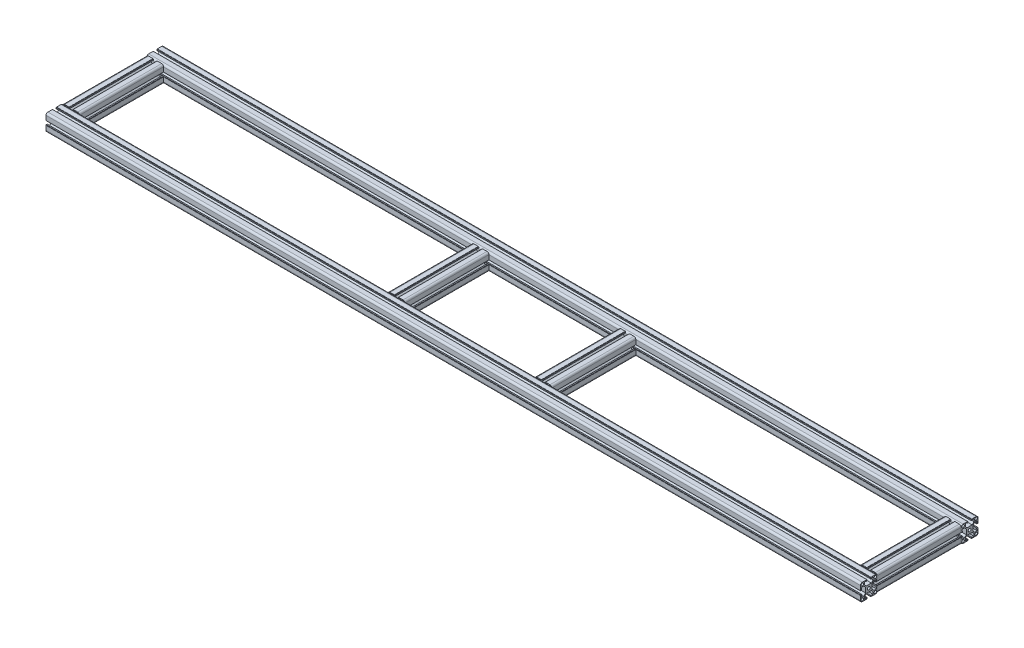
from build123d import *

# Parameters (mm, degrees)
F_40_X_40W_X_R4_5_1_DEPTH      = 1920
F_40_X_40W_X_R4_5_1_DEPTH_BACK = 20
SKETCH1_R                      = 3.4
SKETCH1_R_2                    = 3
SKETCH1_ON_SEGMENT_2_R         = 3.4
SKETCH1_ON_SEGMENT_2_R_2       = 3
F_40_X_40W_X_R4_5_1_2_DEPTH    = 1940
SKETCH1_ON_SEGMENT_3_R         = 3.4
SKETCH1_ON_SEGMENT_3_R_2       = 3
F_40_X_40W_X_R4_5_1_3_DEPTH    = 242
SKETCH1_ON_SEGMENT_4_R         = 3.4
SKETCH1_ON_SEGMENT_4_R_2       = 3
F_40_X_40W_X_R4_5_1_4_DEPTH    = 242
SKETCH1_ON_SEGMENT_5_R         = 3.4
SKETCH1_ON_SEGMENT_5_R_2       = 3
F_40_X_40W_X_R4_5_1_5_DEPTH    = 242
SKETCH1_ON_SEGMENT_6_R         = 3.4
SKETCH1_ON_SEGMENT_6_R_2       = 3
F_40_X_40W_X_R4_5_1_6_DEPTH    = 242


with BuildPart() as part:
    # Sketch1 → 铝型材 40 X 40W X R4.5(1) (new, two sides: drawn at the far end of the back side and taken through both)
    with BuildSketch(Plane(origin=(-950, 0, -120), x_dir=(0, 0, -1), z_dir=(1, 0, 0)).offset(-F_40_X_40W_X_R4_5_1_DEPTH_BACK)):
        with BuildLine():
            Line((-5.1, 20), (-5.1, 19.5))
            Line((-5.1, 19.5), (-4.1, 19.5))
            Line((-4.1, 19.5), (-4.1, 17))
            Line((-4.1, 17), (-6.1, 17))
            Line((-6.1, 17), (-6.1, 18))
            Line((-6.1, 18), (-10.3, 18))
            Line((-10.3, 18), (-10.3, 12))
            Line((-10.3, 12), (-6, 7.7))
            Line((-6, 7.7), (6, 7.7))
            Line((6, 7.7), (10.3, 12))
            Line((10.3, 12), (10.3, 18))
            Line((10.3, 18), (6.1, 18))
            Line((6.1, 18), (6.1, 17))
            Line((6.1, 17), (4.1, 17))
            Line((4.1, 17), (4.1, 19.5))
            Line((4.1, 19.5), (5.1, 19.5))
            Line((5.1, 19.5), (5.1, 20))
            Line((5.1, 20), (15.5, 20))
            ThreePointArc((15.5, 20), (18.681980515, 18.681980515), (20, 15.5))
            Line((20, 15.5), (20, 5.1))
            Line((20, 5.1), (19.5, 5.1))
            Line((19.5, 5.1), (19.5, 4.1))
            Line((19.5, 4.1), (17, 4.1))
            Line((17, 4.1), (17, 6.1))
            Line((17, 6.1), (18, 6.1))
            Line((18, 6.1), (18, 10.3))
            Line((18, 10.3), (12, 10.3))
            Line((12, 10.3), (7.7, 6))
            Line((7.7, 6), (7.7, -6))
            Line((7.7, -6), (12, -10.3))
            Line((12, -10.3), (18, -10.3))
            Line((18, -10.3), (18, -6.1))
            Line((18, -6.1), (17, -6.1))
            Line((17, -6.1), (17, -4.1))
            Line((17, -4.1), (19.5, -4.1))
            Line((19.5, -4.1), (19.5, -5.1))
            Line((19.5, -5.1), (20, -5.1))
            Line((20, -5.1), (20, -15.5))
            ThreePointArc((20, -15.5), (18.681980515, -18.681980515), (15.5, -20))
            Line((15.5, -20), (5.1, -20))
            Line((5.1, -20), (5.1, -19.5))
            Line((5.1, -19.5), (4.1, -19.5))
            Line((4.1, -19.5), (4.1, -17))
            Line((4.1, -17), (6.1, -17))
            Line((6.1, -17), (6.1, -18))
            Line((6.1, -18), (10.3, -18))
            Line((10.3, -18), (10.3, -12))
            Line((10.3, -12), (6, -7.7))
            Line((6, -7.7), (-6, -7.7))
            Line((-6, -7.7), (-10.3, -12))
            Line((-10.3, -12), (-10.3, -18))
            Line((-10.3, -18), (-6.1, -18))
            Line((-6.1, -18), (-6.1, -17))
            Line((-6.1, -17), (-4.1, -17))
            Line((-4.1, -17), (-4.1, -19.5))
            Line((-4.1, -19.5), (-5.1, -19.5))
            Line((-5.1, -19.5), (-5.1, -20))
            Line((-5.1, -20), (-15.5, -20))
            ThreePointArc((-15.5, -20), (-18.681980515, -18.681980515), (-20, -15.5))
            Line((-20, -15.5), (-20, -5.1))
            Line((-20, -5.1), (-19.5, -5.1))
            Line((-19.5, -5.1), (-19.5, -4.1))
            Line((-19.5, -4.1), (-17, -4.1))
            Line((-17, -4.1), (-17, -6.1))
            Line((-17, -6.1), (-18, -6.1))
            Line((-18, -6.1), (-18, -10.3))
            Line((-18, -10.3), (-12, -10.3))
            Line((-12, -10.3), (-7.7, -6))
            Line((-7.7, -6), (-7.7, 6))
            Line((-7.7, 6), (-12, 10.3))
            Line((-12, 10.3), (-18, 10.3))
            Line((-18, 10.3), (-18, 6.1))
            Line((-18, 6.1), (-17, 6.1))
            Line((-17, 6.1), (-17, 4.1))
            Line((-17, 4.1), (-19.5, 4.1))
            Line((-19.5, 4.1), (-19.5, 5.1))
            Line((-19.5, 5.1), (-20, 5.1))
            Line((-20, 5.1), (-20, 15.5))
            ThreePointArc((-20, 15.5), (-18.681980515, 18.681980515), (-15.5, 20))
            Line((-15.5, 20), (-5.1, 20))
        make_face()
        Circle(SKETCH1_R, mode=Mode.SUBTRACT)
        with Locations((-15.556349186, 15.556349186)):
            Circle(SKETCH1_R_2, mode=Mode.SUBTRACT)
        with Locations((15.556349186, 15.556349186)):
            Circle(SKETCH1_R_2, mode=Mode.SUBTRACT)
        with Locations((15.556349186, -15.556349186)):
            Circle(SKETCH1_R_2, mode=Mode.SUBTRACT)
        with Locations((-15.556349186, -15.556349186)):
            Circle(SKETCH1_R_2, mode=Mode.SUBTRACT)
    extrude(amount=F_40_X_40W_X_R4_5_1_DEPTH + F_40_X_40W_X_R4_5_1_DEPTH_BACK)


with BuildPart() as body_2:
    # Sketch1 on segment 2 (carried to segment 2) → 40 X 40W X R4.5_1 2 (new body)
    with BuildSketch(Plane(origin=(-970, 0, 120), x_dir=(0, 0, -1), z_dir=(1, 0, 0))):
        with BuildLine():
            Line((-5.1, 20), (-5.1, 19.5))
            Line((-5.1, 19.5), (-4.1, 19.5))
            Line((-4.1, 19.5), (-4.1, 17))
            Line((-4.1, 17), (-6.1, 17))
            Line((-6.1, 17), (-6.1, 18))
            Line((-6.1, 18), (-10.3, 18))
            Line((-10.3, 18), (-10.3, 12))
            Line((-10.3, 12), (-6, 7.7))
            Line((-6, 7.7), (6, 7.7))
            Line((6, 7.7), (10.3, 12))
            Line((10.3, 12), (10.3, 18))
            Line((10.3, 18), (6.1, 18))
            Line((6.1, 18), (6.1, 17))
            Line((6.1, 17), (4.1, 17))
            Line((4.1, 17), (4.1, 19.5))
            Line((4.1, 19.5), (5.1, 19.5))
            Line((5.1, 19.5), (5.1, 20))
            Line((5.1, 20), (15.5, 20))
            ThreePointArc((15.5, 20), (18.681980515, 18.681980515), (20, 15.5))
            Line((20, 15.5), (20, 5.1))
            Line((20, 5.1), (19.5, 5.1))
            Line((19.5, 5.1), (19.5, 4.1))
            Line((19.5, 4.1), (17, 4.1))
            Line((17, 4.1), (17, 6.1))
            Line((17, 6.1), (18, 6.1))
            Line((18, 6.1), (18, 10.3))
            Line((18, 10.3), (12, 10.3))
            Line((12, 10.3), (7.7, 6))
            Line((7.7, 6), (7.7, -6))
            Line((7.7, -6), (12, -10.3))
            Line((12, -10.3), (18, -10.3))
            Line((18, -10.3), (18, -6.1))
            Line((18, -6.1), (17, -6.1))
            Line((17, -6.1), (17, -4.1))
            Line((17, -4.1), (19.5, -4.1))
            Line((19.5, -4.1), (19.5, -5.1))
            Line((19.5, -5.1), (20, -5.1))
            Line((20, -5.1), (20, -15.5))
            ThreePointArc((20, -15.5), (18.681980515, -18.681980515), (15.5, -20))
            Line((15.5, -20), (5.1, -20))
            Line((5.1, -20), (5.1, -19.5))
            Line((5.1, -19.5), (4.1, -19.5))
            Line((4.1, -19.5), (4.1, -17))
            Line((4.1, -17), (6.1, -17))
            Line((6.1, -17), (6.1, -18))
            Line((6.1, -18), (10.3, -18))
            Line((10.3, -18), (10.3, -12))
            Line((10.3, -12), (6, -7.7))
            Line((6, -7.7), (-6, -7.7))
            Line((-6, -7.7), (-10.3, -12))
            Line((-10.3, -12), (-10.3, -18))
            Line((-10.3, -18), (-6.1, -18))
            Line((-6.1, -18), (-6.1, -17))
            Line((-6.1, -17), (-4.1, -17))
            Line((-4.1, -17), (-4.1, -19.5))
            Line((-4.1, -19.5), (-5.1, -19.5))
            Line((-5.1, -19.5), (-5.1, -20))
            Line((-5.1, -20), (-15.5, -20))
            ThreePointArc((-15.5, -20), (-18.681980515, -18.681980515), (-20, -15.5))
            Line((-20, -15.5), (-20, -5.1))
            Line((-20, -5.1), (-19.5, -5.1))
            Line((-19.5, -5.1), (-19.5, -4.1))
            Line((-19.5, -4.1), (-17, -4.1))
            Line((-17, -4.1), (-17, -6.1))
            Line((-17, -6.1), (-18, -6.1))
            Line((-18, -6.1), (-18, -10.3))
            Line((-18, -10.3), (-12, -10.3))
            Line((-12, -10.3), (-7.7, -6))
            Line((-7.7, -6), (-7.7, 6))
            Line((-7.7, 6), (-12, 10.3))
            Line((-12, 10.3), (-18, 10.3))
            Line((-18, 10.3), (-18, 6.1))
            Line((-18, 6.1), (-17, 6.1))
            Line((-17, 6.1), (-17, 4.1))
            Line((-17, 4.1), (-19.5, 4.1))
            Line((-19.5, 4.1), (-19.5, 5.1))
            Line((-19.5, 5.1), (-20, 5.1))
            Line((-20, 5.1), (-20, 15.5))
            ThreePointArc((-20, 15.5), (-18.681980515, 18.681980515), (-15.5, 20))
            Line((-15.5, 20), (-5.1, 20))
        make_face()
        Circle(SKETCH1_ON_SEGMENT_2_R, mode=Mode.SUBTRACT)
        with Locations((-15.556349186, 15.556349186)):
            Circle(SKETCH1_ON_SEGMENT_2_R_2, mode=Mode.SUBTRACT)
        with Locations((15.556349186, 15.556349186)):
            Circle(SKETCH1_ON_SEGMENT_2_R_2, mode=Mode.SUBTRACT)
        with Locations((15.556349186, -15.556349186)):
            Circle(SKETCH1_ON_SEGMENT_2_R_2, mode=Mode.SUBTRACT)
        with Locations((-15.556349186, -15.556349186)):
            Circle(SKETCH1_ON_SEGMENT_2_R_2, mode=Mode.SUBTRACT)
    extrude(amount=F_40_X_40W_X_R4_5_1_2_DEPTH)


with BuildPart() as body_3:
    # Sketch1 on segment 3 (carried to segment 3) → 40 X 40W X R4.5_1 3 (new body)
    with BuildSketch(Plane(origin=(-950, 0, -121), x_dir=(1, 0, 0), z_dir=(0, 0, 1))):
        with BuildLine():
            Line((-5.1, 20), (-5.1, 19.5))
            Line((-5.1, 19.5), (-4.1, 19.5))
            Line((-4.1, 19.5), (-4.1, 17))
            Line((-4.1, 17), (-6.1, 17))
            Line((-6.1, 17), (-6.1, 18))
            Line((-6.1, 18), (-10.3, 18))
            Line((-10.3, 18), (-10.3, 12))
            Line((-10.3, 12), (-6, 7.7))
            Line((-6, 7.7), (6, 7.7))
            Line((6, 7.7), (10.3, 12))
            Line((10.3, 12), (10.3, 18))
            Line((10.3, 18), (6.1, 18))
            Line((6.1, 18), (6.1, 17))
            Line((6.1, 17), (4.1, 17))
            Line((4.1, 17), (4.1, 19.5))
            Line((4.1, 19.5), (5.1, 19.5))
            Line((5.1, 19.5), (5.1, 20))
            Line((5.1, 20), (15.5, 20))
            ThreePointArc((15.5, 20), (18.681980515, 18.681980515), (20, 15.5))
            Line((20, 15.5), (20, 5.1))
            Line((20, 5.1), (19.5, 5.1))
            Line((19.5, 5.1), (19.5, 4.1))
            Line((19.5, 4.1), (17, 4.1))
            Line((17, 4.1), (17, 6.1))
            Line((17, 6.1), (18, 6.1))
            Line((18, 6.1), (18, 10.3))
            Line((18, 10.3), (12, 10.3))
            Line((12, 10.3), (7.7, 6))
            Line((7.7, 6), (7.7, -6))
            Line((7.7, -6), (12, -10.3))
            Line((12, -10.3), (18, -10.3))
            Line((18, -10.3), (18, -6.1))
            Line((18, -6.1), (17, -6.1))
            Line((17, -6.1), (17, -4.1))
            Line((17, -4.1), (19.5, -4.1))
            Line((19.5, -4.1), (19.5, -5.1))
            Line((19.5, -5.1), (20, -5.1))
            Line((20, -5.1), (20, -15.5))
            ThreePointArc((20, -15.5), (18.681980515, -18.681980515), (15.5, -20))
            Line((15.5, -20), (5.1, -20))
            Line((5.1, -20), (5.1, -19.5))
            Line((5.1, -19.5), (4.1, -19.5))
            Line((4.1, -19.5), (4.1, -17))
            Line((4.1, -17), (6.1, -17))
            Line((6.1, -17), (6.1, -18))
            Line((6.1, -18), (10.3, -18))
            Line((10.3, -18), (10.3, -12))
            Line((10.3, -12), (6, -7.7))
            Line((6, -7.7), (-6, -7.7))
            Line((-6, -7.7), (-10.3, -12))
            Line((-10.3, -12), (-10.3, -18))
            Line((-10.3, -18), (-6.1, -18))
            Line((-6.1, -18), (-6.1, -17))
            Line((-6.1, -17), (-4.1, -17))
            Line((-4.1, -17), (-4.1, -19.5))
            Line((-4.1, -19.5), (-5.1, -19.5))
            Line((-5.1, -19.5), (-5.1, -20))
            Line((-5.1, -20), (-15.5, -20))
            ThreePointArc((-15.5, -20), (-18.681980515, -18.681980515), (-20, -15.5))
            Line((-20, -15.5), (-20, -5.1))
            Line((-20, -5.1), (-19.5, -5.1))
            Line((-19.5, -5.1), (-19.5, -4.1))
            Line((-19.5, -4.1), (-17, -4.1))
            Line((-17, -4.1), (-17, -6.1))
            Line((-17, -6.1), (-18, -6.1))
            Line((-18, -6.1), (-18, -10.3))
            Line((-18, -10.3), (-12, -10.3))
            Line((-12, -10.3), (-7.7, -6))
            Line((-7.7, -6), (-7.7, 6))
            Line((-7.7, 6), (-12, 10.3))
            Line((-12, 10.3), (-18, 10.3))
            Line((-18, 10.3), (-18, 6.1))
            Line((-18, 6.1), (-17, 6.1))
            Line((-17, 6.1), (-17, 4.1))
            Line((-17, 4.1), (-19.5, 4.1))
            Line((-19.5, 4.1), (-19.5, 5.1))
            Line((-19.5, 5.1), (-20, 5.1))
            Line((-20, 5.1), (-20, 15.5))
            ThreePointArc((-20, 15.5), (-18.681980515, 18.681980515), (-15.5, 20))
            Line((-15.5, 20), (-5.1, 20))
        make_face()
        Circle(SKETCH1_ON_SEGMENT_3_R, mode=Mode.SUBTRACT)
        with Locations((-15.556349186, 15.556349186)):
            Circle(SKETCH1_ON_SEGMENT_3_R_2, mode=Mode.SUBTRACT)
        with Locations((15.556349186, 15.556349186)):
            Circle(SKETCH1_ON_SEGMENT_3_R_2, mode=Mode.SUBTRACT)
        with Locations((15.556349186, -15.556349186)):
            Circle(SKETCH1_ON_SEGMENT_3_R_2, mode=Mode.SUBTRACT)
        with Locations((-15.556349186, -15.556349186)):
            Circle(SKETCH1_ON_SEGMENT_3_R_2, mode=Mode.SUBTRACT)
    extrude(amount=F_40_X_40W_X_R4_5_1_3_DEPTH)

    # 40 X 40W X R4.5_1 3 end butt 1
    split(bisect_by=Plane(origin=(-950, 0, -100), x_dir=(0, -1, 0), z_dir=(0, 0, 1)), keep=Keep.TOP)

    # 40 X 40W X R4.5_1 3 end butt 2
    split(bisect_by=Plane(origin=(-950, 0, 100), x_dir=(0, 1, 0), z_dir=(0, 0, -1)), keep=Keep.TOP)


with BuildPart() as body_4:
    # Sketch1 on segment 4 (carried to segment 4) → 40 X 40W X R4.5_1 4 (new body)
    with BuildSketch(Plane(origin=(-175, 0, -121), x_dir=(1, 0, 0), z_dir=(0, 0, 1))):
        with BuildLine():
            Line((-5.1, 20), (-5.1, 19.5))
            Line((-5.1, 19.5), (-4.1, 19.5))
            Line((-4.1, 19.5), (-4.1, 17))
            Line((-4.1, 17), (-6.1, 17))
            Line((-6.1, 17), (-6.1, 18))
            Line((-6.1, 18), (-10.3, 18))
            Line((-10.3, 18), (-10.3, 12))
            Line((-10.3, 12), (-6, 7.7))
            Line((-6, 7.7), (6, 7.7))
            Line((6, 7.7), (10.3, 12))
            Line((10.3, 12), (10.3, 18))
            Line((10.3, 18), (6.1, 18))
            Line((6.1, 18), (6.1, 17))
            Line((6.1, 17), (4.1, 17))
            Line((4.1, 17), (4.1, 19.5))
            Line((4.1, 19.5), (5.1, 19.5))
            Line((5.1, 19.5), (5.1, 20))
            Line((5.1, 20), (15.5, 20))
            ThreePointArc((15.5, 20), (18.681980515, 18.681980515), (20, 15.5))
            Line((20, 15.5), (20, 5.1))
            Line((20, 5.1), (19.5, 5.1))
            Line((19.5, 5.1), (19.5, 4.1))
            Line((19.5, 4.1), (17, 4.1))
            Line((17, 4.1), (17, 6.1))
            Line((17, 6.1), (18, 6.1))
            Line((18, 6.1), (18, 10.3))
            Line((18, 10.3), (12, 10.3))
            Line((12, 10.3), (7.7, 6))
            Line((7.7, 6), (7.7, -6))
            Line((7.7, -6), (12, -10.3))
            Line((12, -10.3), (18, -10.3))
            Line((18, -10.3), (18, -6.1))
            Line((18, -6.1), (17, -6.1))
            Line((17, -6.1), (17, -4.1))
            Line((17, -4.1), (19.5, -4.1))
            Line((19.5, -4.1), (19.5, -5.1))
            Line((19.5, -5.1), (20, -5.1))
            Line((20, -5.1), (20, -15.5))
            ThreePointArc((20, -15.5), (18.681980515, -18.681980515), (15.5, -20))
            Line((15.5, -20), (5.1, -20))
            Line((5.1, -20), (5.1, -19.5))
            Line((5.1, -19.5), (4.1, -19.5))
            Line((4.1, -19.5), (4.1, -17))
            Line((4.1, -17), (6.1, -17))
            Line((6.1, -17), (6.1, -18))
            Line((6.1, -18), (10.3, -18))
            Line((10.3, -18), (10.3, -12))
            Line((10.3, -12), (6, -7.7))
            Line((6, -7.7), (-6, -7.7))
            Line((-6, -7.7), (-10.3, -12))
            Line((-10.3, -12), (-10.3, -18))
            Line((-10.3, -18), (-6.1, -18))
            Line((-6.1, -18), (-6.1, -17))
            Line((-6.1, -17), (-4.1, -17))
            Line((-4.1, -17), (-4.1, -19.5))
            Line((-4.1, -19.5), (-5.1, -19.5))
            Line((-5.1, -19.5), (-5.1, -20))
            Line((-5.1, -20), (-15.5, -20))
            ThreePointArc((-15.5, -20), (-18.681980515, -18.681980515), (-20, -15.5))
            Line((-20, -15.5), (-20, -5.1))
            Line((-20, -5.1), (-19.5, -5.1))
            Line((-19.5, -5.1), (-19.5, -4.1))
            Line((-19.5, -4.1), (-17, -4.1))
            Line((-17, -4.1), (-17, -6.1))
            Line((-17, -6.1), (-18, -6.1))
            Line((-18, -6.1), (-18, -10.3))
            Line((-18, -10.3), (-12, -10.3))
            Line((-12, -10.3), (-7.7, -6))
            Line((-7.7, -6), (-7.7, 6))
            Line((-7.7, 6), (-12, 10.3))
            Line((-12, 10.3), (-18, 10.3))
            Line((-18, 10.3), (-18, 6.1))
            Line((-18, 6.1), (-17, 6.1))
            Line((-17, 6.1), (-17, 4.1))
            Line((-17, 4.1), (-19.5, 4.1))
            Line((-19.5, 4.1), (-19.5, 5.1))
            Line((-19.5, 5.1), (-20, 5.1))
            Line((-20, 5.1), (-20, 15.5))
            ThreePointArc((-20, 15.5), (-18.681980515, 18.681980515), (-15.5, 20))
            Line((-15.5, 20), (-5.1, 20))
        make_face()
        Circle(SKETCH1_ON_SEGMENT_4_R, mode=Mode.SUBTRACT)
        with Locations((-15.556349186, 15.556349186)):
            Circle(SKETCH1_ON_SEGMENT_4_R_2, mode=Mode.SUBTRACT)
        with Locations((15.556349186, 15.556349186)):
            Circle(SKETCH1_ON_SEGMENT_4_R_2, mode=Mode.SUBTRACT)
        with Locations((15.556349186, -15.556349186)):
            Circle(SKETCH1_ON_SEGMENT_4_R_2, mode=Mode.SUBTRACT)
        with Locations((-15.556349186, -15.556349186)):
            Circle(SKETCH1_ON_SEGMENT_4_R_2, mode=Mode.SUBTRACT)
    extrude(amount=F_40_X_40W_X_R4_5_1_4_DEPTH)

    # 40 X 40W X R4.5_1 4 end butt 1
    split(bisect_by=Plane(origin=(-175, 0, -100), x_dir=(0, -1, 0), z_dir=(0, 0, 1)), keep=Keep.TOP)

    # 40 X 40W X R4.5_1 4 end butt 2
    split(bisect_by=Plane(origin=(-175, 0, 100), x_dir=(0, 1, 0), z_dir=(0, 0, -1)), keep=Keep.TOP)


with BuildPart() as body_5:
    # Sketch1 on segment 5 (carried to segment 5) → 40 X 40W X R4.5_1 5 (new body)
    with BuildSketch(Plane(origin=(175, 0, -121), x_dir=(1, 0, 0), z_dir=(0, 0, 1))):
        with BuildLine():
            Line((-5.1, 20), (-5.1, 19.5))
            Line((-5.1, 19.5), (-4.1, 19.5))
            Line((-4.1, 19.5), (-4.1, 17))
            Line((-4.1, 17), (-6.1, 17))
            Line((-6.1, 17), (-6.1, 18))
            Line((-6.1, 18), (-10.3, 18))
            Line((-10.3, 18), (-10.3, 12))
            Line((-10.3, 12), (-6, 7.7))
            Line((-6, 7.7), (6, 7.7))
            Line((6, 7.7), (10.3, 12))
            Line((10.3, 12), (10.3, 18))
            Line((10.3, 18), (6.1, 18))
            Line((6.1, 18), (6.1, 17))
            Line((6.1, 17), (4.1, 17))
            Line((4.1, 17), (4.1, 19.5))
            Line((4.1, 19.5), (5.1, 19.5))
            Line((5.1, 19.5), (5.1, 20))
            Line((5.1, 20), (15.5, 20))
            ThreePointArc((15.5, 20), (18.681980515, 18.681980515), (20, 15.5))
            Line((20, 15.5), (20, 5.1))
            Line((20, 5.1), (19.5, 5.1))
            Line((19.5, 5.1), (19.5, 4.1))
            Line((19.5, 4.1), (17, 4.1))
            Line((17, 4.1), (17, 6.1))
            Line((17, 6.1), (18, 6.1))
            Line((18, 6.1), (18, 10.3))
            Line((18, 10.3), (12, 10.3))
            Line((12, 10.3), (7.7, 6))
            Line((7.7, 6), (7.7, -6))
            Line((7.7, -6), (12, -10.3))
            Line((12, -10.3), (18, -10.3))
            Line((18, -10.3), (18, -6.1))
            Line((18, -6.1), (17, -6.1))
            Line((17, -6.1), (17, -4.1))
            Line((17, -4.1), (19.5, -4.1))
            Line((19.5, -4.1), (19.5, -5.1))
            Line((19.5, -5.1), (20, -5.1))
            Line((20, -5.1), (20, -15.5))
            ThreePointArc((20, -15.5), (18.681980515, -18.681980515), (15.5, -20))
            Line((15.5, -20), (5.1, -20))
            Line((5.1, -20), (5.1, -19.5))
            Line((5.1, -19.5), (4.1, -19.5))
            Line((4.1, -19.5), (4.1, -17))
            Line((4.1, -17), (6.1, -17))
            Line((6.1, -17), (6.1, -18))
            Line((6.1, -18), (10.3, -18))
            Line((10.3, -18), (10.3, -12))
            Line((10.3, -12), (6, -7.7))
            Line((6, -7.7), (-6, -7.7))
            Line((-6, -7.7), (-10.3, -12))
            Line((-10.3, -12), (-10.3, -18))
            Line((-10.3, -18), (-6.1, -18))
            Line((-6.1, -18), (-6.1, -17))
            Line((-6.1, -17), (-4.1, -17))
            Line((-4.1, -17), (-4.1, -19.5))
            Line((-4.1, -19.5), (-5.1, -19.5))
            Line((-5.1, -19.5), (-5.1, -20))
            Line((-5.1, -20), (-15.5, -20))
            ThreePointArc((-15.5, -20), (-18.681980515, -18.681980515), (-20, -15.5))
            Line((-20, -15.5), (-20, -5.1))
            Line((-20, -5.1), (-19.5, -5.1))
            Line((-19.5, -5.1), (-19.5, -4.1))
            Line((-19.5, -4.1), (-17, -4.1))
            Line((-17, -4.1), (-17, -6.1))
            Line((-17, -6.1), (-18, -6.1))
            Line((-18, -6.1), (-18, -10.3))
            Line((-18, -10.3), (-12, -10.3))
            Line((-12, -10.3), (-7.7, -6))
            Line((-7.7, -6), (-7.7, 6))
            Line((-7.7, 6), (-12, 10.3))
            Line((-12, 10.3), (-18, 10.3))
            Line((-18, 10.3), (-18, 6.1))
            Line((-18, 6.1), (-17, 6.1))
            Line((-17, 6.1), (-17, 4.1))
            Line((-17, 4.1), (-19.5, 4.1))
            Line((-19.5, 4.1), (-19.5, 5.1))
            Line((-19.5, 5.1), (-20, 5.1))
            Line((-20, 5.1), (-20, 15.5))
            ThreePointArc((-20, 15.5), (-18.681980515, 18.681980515), (-15.5, 20))
            Line((-15.5, 20), (-5.1, 20))
        make_face()
        Circle(SKETCH1_ON_SEGMENT_5_R, mode=Mode.SUBTRACT)
        with Locations((-15.556349186, 15.556349186)):
            Circle(SKETCH1_ON_SEGMENT_5_R_2, mode=Mode.SUBTRACT)
        with Locations((15.556349186, 15.556349186)):
            Circle(SKETCH1_ON_SEGMENT_5_R_2, mode=Mode.SUBTRACT)
        with Locations((15.556349186, -15.556349186)):
            Circle(SKETCH1_ON_SEGMENT_5_R_2, mode=Mode.SUBTRACT)
        with Locations((-15.556349186, -15.556349186)):
            Circle(SKETCH1_ON_SEGMENT_5_R_2, mode=Mode.SUBTRACT)
    extrude(amount=F_40_X_40W_X_R4_5_1_5_DEPTH)

    # 40 X 40W X R4.5_1 5 end butt 1
    split(bisect_by=Plane(origin=(175, 0, -100), x_dir=(0, -1, 0), z_dir=(0, 0, 1)), keep=Keep.TOP)

    # 40 X 40W X R4.5_1 5 end butt 2
    split(bisect_by=Plane(origin=(175, 0, 100), x_dir=(0, 1, 0), z_dir=(0, 0, -1)), keep=Keep.TOP)


with BuildPart() as body_6:
    # Sketch1 on segment 6 (carried to segment 6) → 40 X 40W X R4.5_1 6 (new body)
    with BuildSketch(Plane(origin=(950, 0, -121), x_dir=(1, 0, 0), z_dir=(0, 0, 1))):
        with BuildLine():
            Line((-5.1, 20), (-5.1, 19.5))
            Line((-5.1, 19.5), (-4.1, 19.5))
            Line((-4.1, 19.5), (-4.1, 17))
            Line((-4.1, 17), (-6.1, 17))
            Line((-6.1, 17), (-6.1, 18))
            Line((-6.1, 18), (-10.3, 18))
            Line((-10.3, 18), (-10.3, 12))
            Line((-10.3, 12), (-6, 7.7))
            Line((-6, 7.7), (6, 7.7))
            Line((6, 7.7), (10.3, 12))
            Line((10.3, 12), (10.3, 18))
            Line((10.3, 18), (6.1, 18))
            Line((6.1, 18), (6.1, 17))
            Line((6.1, 17), (4.1, 17))
            Line((4.1, 17), (4.1, 19.5))
            Line((4.1, 19.5), (5.1, 19.5))
            Line((5.1, 19.5), (5.1, 20))
            Line((5.1, 20), (15.5, 20))
            ThreePointArc((15.5, 20), (18.681980515, 18.681980515), (20, 15.5))
            Line((20, 15.5), (20, 5.1))
            Line((20, 5.1), (19.5, 5.1))
            Line((19.5, 5.1), (19.5, 4.1))
            Line((19.5, 4.1), (17, 4.1))
            Line((17, 4.1), (17, 6.1))
            Line((17, 6.1), (18, 6.1))
            Line((18, 6.1), (18, 10.3))
            Line((18, 10.3), (12, 10.3))
            Line((12, 10.3), (7.7, 6))
            Line((7.7, 6), (7.7, -6))
            Line((7.7, -6), (12, -10.3))
            Line((12, -10.3), (18, -10.3))
            Line((18, -10.3), (18, -6.1))
            Line((18, -6.1), (17, -6.1))
            Line((17, -6.1), (17, -4.1))
            Line((17, -4.1), (19.5, -4.1))
            Line((19.5, -4.1), (19.5, -5.1))
            Line((19.5, -5.1), (20, -5.1))
            Line((20, -5.1), (20, -15.5))
            ThreePointArc((20, -15.5), (18.681980515, -18.681980515), (15.5, -20))
            Line((15.5, -20), (5.1, -20))
            Line((5.1, -20), (5.1, -19.5))
            Line((5.1, -19.5), (4.1, -19.5))
            Line((4.1, -19.5), (4.1, -17))
            Line((4.1, -17), (6.1, -17))
            Line((6.1, -17), (6.1, -18))
            Line((6.1, -18), (10.3, -18))
            Line((10.3, -18), (10.3, -12))
            Line((10.3, -12), (6, -7.7))
            Line((6, -7.7), (-6, -7.7))
            Line((-6, -7.7), (-10.3, -12))
            Line((-10.3, -12), (-10.3, -18))
            Line((-10.3, -18), (-6.1, -18))
            Line((-6.1, -18), (-6.1, -17))
            Line((-6.1, -17), (-4.1, -17))
            Line((-4.1, -17), (-4.1, -19.5))
            Line((-4.1, -19.5), (-5.1, -19.5))
            Line((-5.1, -19.5), (-5.1, -20))
            Line((-5.1, -20), (-15.5, -20))
            ThreePointArc((-15.5, -20), (-18.681980515, -18.681980515), (-20, -15.5))
            Line((-20, -15.5), (-20, -5.1))
            Line((-20, -5.1), (-19.5, -5.1))
            Line((-19.5, -5.1), (-19.5, -4.1))
            Line((-19.5, -4.1), (-17, -4.1))
            Line((-17, -4.1), (-17, -6.1))
            Line((-17, -6.1), (-18, -6.1))
            Line((-18, -6.1), (-18, -10.3))
            Line((-18, -10.3), (-12, -10.3))
            Line((-12, -10.3), (-7.7, -6))
            Line((-7.7, -6), (-7.7, 6))
            Line((-7.7, 6), (-12, 10.3))
            Line((-12, 10.3), (-18, 10.3))
            Line((-18, 10.3), (-18, 6.1))
            Line((-18, 6.1), (-17, 6.1))
            Line((-17, 6.1), (-17, 4.1))
            Line((-17, 4.1), (-19.5, 4.1))
            Line((-19.5, 4.1), (-19.5, 5.1))
            Line((-19.5, 5.1), (-20, 5.1))
            Line((-20, 5.1), (-20, 15.5))
            ThreePointArc((-20, 15.5), (-18.681980515, 18.681980515), (-15.5, 20))
            Line((-15.5, 20), (-5.1, 20))
        make_face()
        Circle(SKETCH1_ON_SEGMENT_6_R, mode=Mode.SUBTRACT)
        with Locations((-15.556349186, 15.556349186)):
            Circle(SKETCH1_ON_SEGMENT_6_R_2, mode=Mode.SUBTRACT)
        with Locations((15.556349186, 15.556349186)):
            Circle(SKETCH1_ON_SEGMENT_6_R_2, mode=Mode.SUBTRACT)
        with Locations((15.556349186, -15.556349186)):
            Circle(SKETCH1_ON_SEGMENT_6_R_2, mode=Mode.SUBTRACT)
        with Locations((-15.556349186, -15.556349186)):
            Circle(SKETCH1_ON_SEGMENT_6_R_2, mode=Mode.SUBTRACT)
    extrude(amount=F_40_X_40W_X_R4_5_1_6_DEPTH)

    # 40 X 40W X R4.5_1 6 end butt 1
    split(bisect_by=Plane(origin=(950, 0, -100), x_dir=(0, -1, 0), z_dir=(0, 0, 1)), keep=Keep.TOP)

    # 40 X 40W X R4.5_1 6 end butt 2
    split(bisect_by=Plane(origin=(950, 0, 100), x_dir=(0, 1, 0), z_dir=(0, 0, -1)), keep=Keep.TOP)


solid = Compound([part.part, body_2.part, body_3.part, body_4.part, body_5.part, body_6.part])
